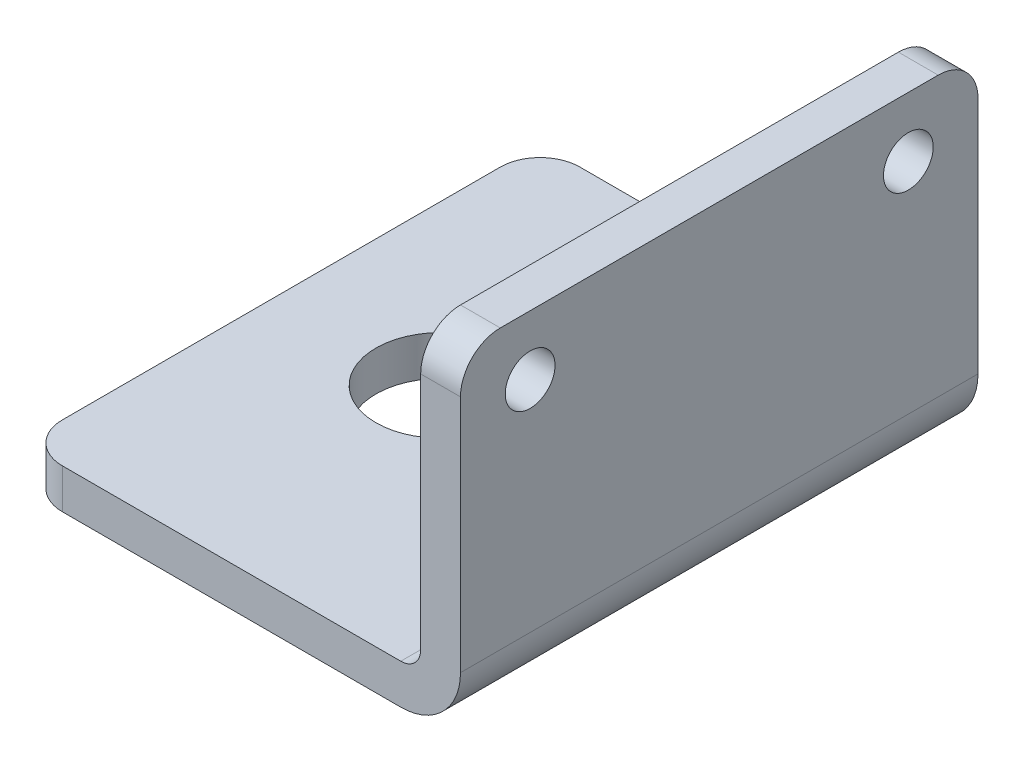
SolidWorks part; units mm, degrees
ref_plane "前视" through (0, 0, 0) normal (0, 0, 1) x (1, 0, 0)
ref_plane "上视" through (0, 0, 0) normal (0, 1, 0) x (1, 0, 0)
ref_plane "右视" through (0, 0, 0) normal (1, 0, 0) x (0, 0, -1)
sketch "草图1" plane through (0, 0, 0) normal (0, 0, 1) x (1, 0, 0)
  line L0 (0, 0) -> (20, 0)
  line L1 (20, 0) -> (20, 15)
  dimension "D1" = 15
  dimension "D2" = 20
extrude "拉伸-薄壁1" add sketch "草图1" along normal blind 26 thin
fillet "圆角1" radius 1 1 edges at (20, 0, 13)
fillet "圆角2" radius 3 1 edges at (22, -2, 13)
fillet "圆角3" radius 2 4 edges at (0, -1, 26) (0, -1, 0) (21, 15, 0) (21, 15, 26)
sketch "草图2" plane through (0, 0, 0) normal (0, 1, 0) x (1, 0, 0)
  line L0 (0, -13) -> (8, -13) construction
  line L1 (0, -24) -> (0, -2) construction
  circle A0 centre (8, -13) radius 3.25
  dimension "D2" = 6.5
  dimension "D1" = 8
extrude "切除-拉伸1" cut sketch "草图2" against normal through all
hole_wizard "M3 螺纹孔1" positions "草图4" profile "草图3" tap size "M3" standard "GB" end condition through all
sketch "草图4" plane through (22, 0, 0) normal (1, 0, 0) x (0, 0, -1)
  line L0 (-13, -2) -> (-13, 29.789) construction
  line L1 (0, -2) -> (-26, -2) construction
  line L3 (-24, 15) -> (-2, 15) construction
  point P0 (-22.5, 12)
  point P3 (-3.5, 12)
  dimension "D1" = 19
  dimension "D2" = 3
sketch "草图3" plane through (22, 12, 22.5) normal (0, 1, 0) x (0, 0, -1)
  line L0 (0, 0) -> (0, 22)
  line L1 (0, 22) -> (1.25, 22)
  line L2 (1.25, 22) -> (1.25, 0)
  line L5 (1.25, 0) -> (0, 0)
  line L11 (0, -6.35) -> (0, 107.95) construction
  dimension "通孔螺纹孔钻头直径" = 2.5
  dimension "通孔螺纹孔钻头深度" = 22
cosmetic thread "孔螺蚊线1" parameters "D2"=3
cosmetic thread "孔螺蚊线2" parameters "D2"=3
